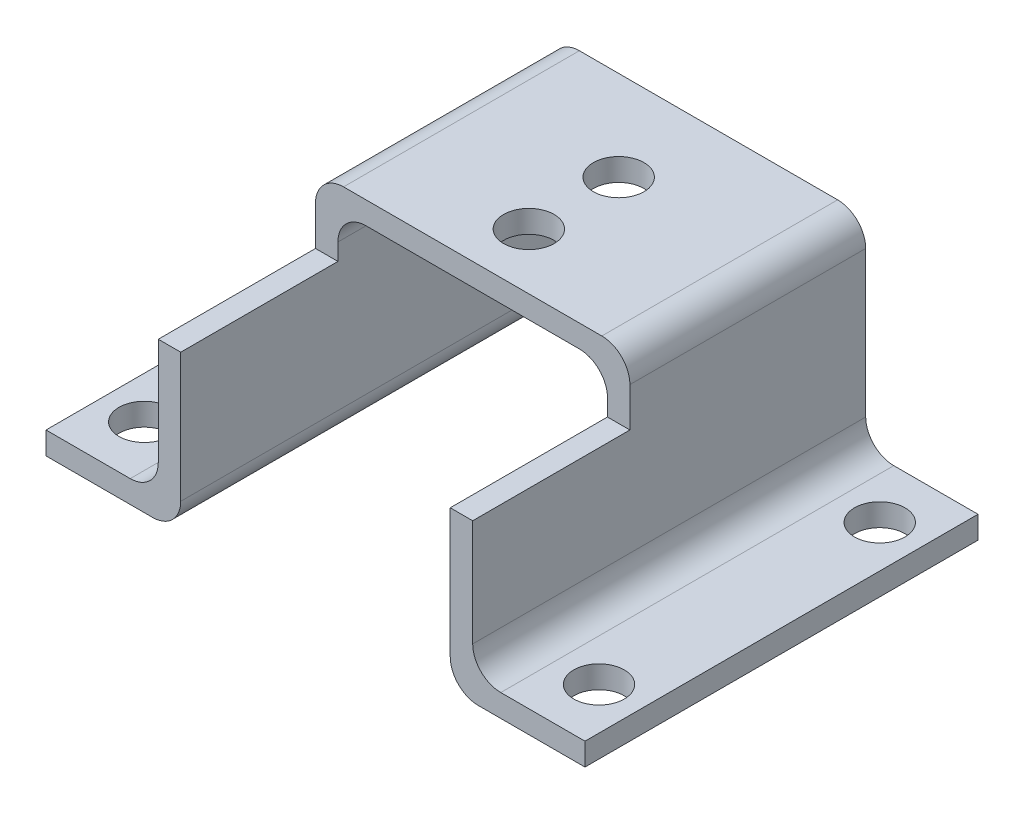
from build123d import *

# Parameters (mm, degrees)
BOSS_EXTRUDE1_DEPTH = 35
SKETCH2_W           = 34.392896322
SKETCH2_H           = 15.037586703
CUT_EXTRUDE1_DEPTH  = 14
SKETCH3_R           = 2.25
CUT_EXTRUDE2_DEPTH  = 19


with BuildPart() as part:
    # Sketch1 → Boss-Extrude1 (new body)
    with BuildSketch(Plane.XY):
        with BuildLine():
            Line((-24, 0), (-14.5, 0))
            ThreePointArc((-14.5, 0), (-12.732233047, 0.732233047), (-12, 2.5))
            Line((-12, 2.5), (-12, 15.5))
            ThreePointArc((-12, 15.5), (-11.267766953, 17.267766953), (-9.5, 18))
            Line((-9.5, 18), (9.5, 18))
            ThreePointArc((9.5, 18), (11.267766953, 17.267766953), (12, 15.5))
            Line((12, 15.5), (12, 2.5))
            ThreePointArc((12, 2.5), (12.732233047, 0.732233047), (14.5, 0))
            Line((14.5, 0), (24, 0))
            Line((24, 0), (24, 2))
            Line((24, 2), (16.5, 2))
            ThreePointArc((16.5, 2), (14.732233047, 2.732233047), (14, 4.5))
            Line((14, 4.5), (14, 17.5))
            ThreePointArc((14, 17.5), (13.267766953, 19.267766953), (11.5, 20))
            Line((11.5, 20), (-11.5, 20))
            ThreePointArc((-11.5, 20), (-13.267766953, 19.267766953), (-14, 17.5))
            Line((-14, 17.5), (-14, 4.5))
            ThreePointArc((-14, 4.5), (-14.732233047, 2.732233047), (-16.5, 2))
            Line((-16.5, 2), (-24, 2))
            Line((-24, 2), (-24, 0))
        make_face()
    extrude(amount=BOSS_EXTRUDE1_DEPTH)

    # Sketch2 → Cut-Extrude1 (cut)
    with BuildSketch(Plane.XY.offset(35)):
        with Locations((0, 21.518793352)):
            Rectangle(SKETCH2_W, SKETCH2_H)
    extrude(amount=-CUT_EXTRUDE1_DEPTH, mode=Mode.SUBTRACT)

    # Sketch3 → Cut-Extrude2 (cut, symmetric)
    with BuildSketch(Plane(origin=(0, 2, 0), x_dir=(1, 0, 0), z_dir=(0, 1, 0))):
        with Locations(Location((-20.25, -5, 0), (0, 0, 90))):
            Circle(SKETCH3_R)
        with Locations(Location((-20.25, -30, 0), (0, 0, 90))):
            Circle(SKETCH3_R)
        with Locations(Location((20.25, -30, 0), (0, 0, 90))):
            Circle(SKETCH3_R)
        with Locations(Location((20.25, -5, 0), (0, 0, 90))):
            Circle(SKETCH3_R)
        with Locations(Location((0, -8, 0), (0, 0, 90))):
            Circle(SKETCH3_R)
        with Locations(Location((0, -16, 0), (0, 0, 90))):
            Circle(SKETCH3_R)
    extrude(amount=CUT_EXTRUDE2_DEPTH, both=True, mode=Mode.SUBTRACT)


solid = part.part
